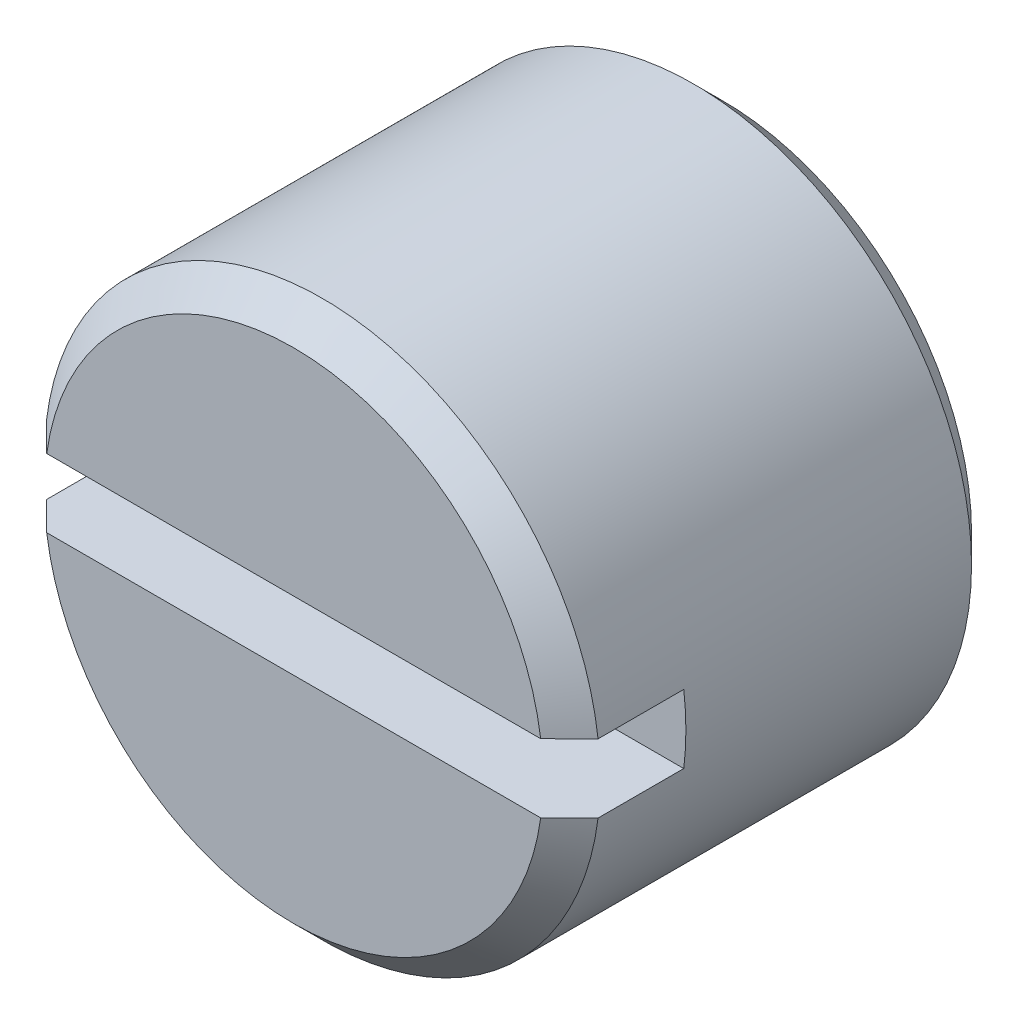
from build123d import *

# Parameters (mm, degrees)
SKETCH1_R           = 4.865
BOSS_EXTRUDE1_DEPTH = 7.5
SKETCH2_W           = 12.82033658
SKETCH2_H           = 1.2
CUT_EXTRUDE1_DEPTH  = 2
CHAMFER1_SIZE       = 0.5


with BuildPart() as part:
    # Sketch1 → Boss-Extrude1 (new body)
    with BuildSketch(Plane.XY):
        Circle(SKETCH1_R)
    extrude(amount=BOSS_EXTRUDE1_DEPTH)

    # Sketch2 → Cut-Extrude1 (cut)
    with BuildSketch(Plane.XY.offset(7.5)):
        Rectangle(SKETCH2_W, SKETCH2_H)
    extrude(amount=-CUT_EXTRUDE1_DEPTH, mode=Mode.SUBTRACT)

    # Chamfer1
    chamfer1_edges = [part.edges().sort_by_distance(p)[0] for p in [
        (-4.865, 0, 0),
        (0, 4.865, 7.5),
        (0, -4.865, 7.5),
    ]]
    chamfer(chamfer1_edges, length=CHAMFER1_SIZE)


solid = part.part
